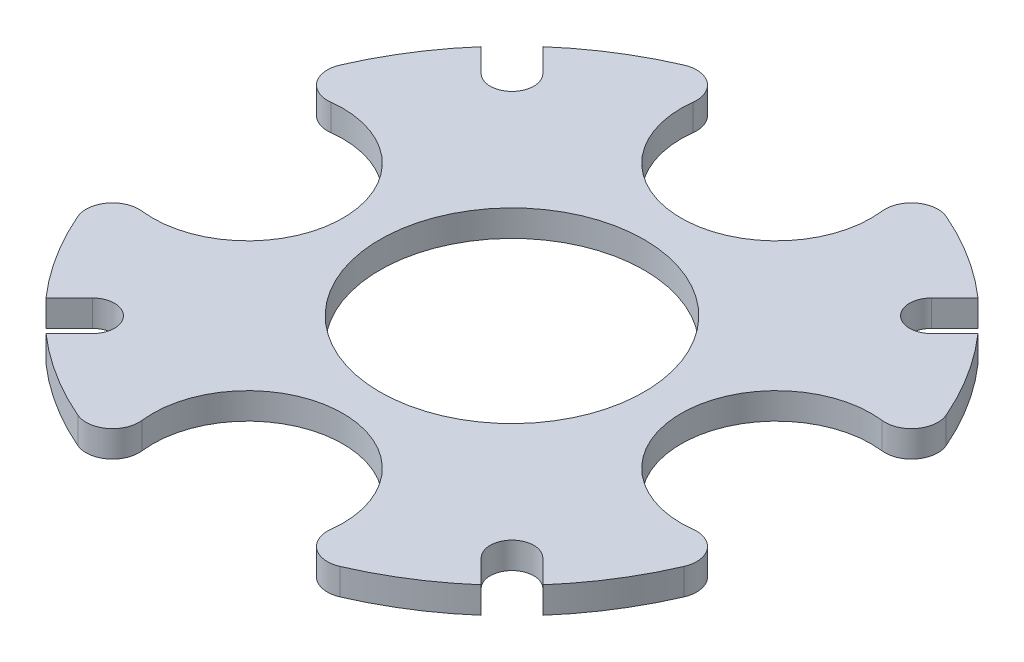
SolidWorks part; units mm, degrees
material "201 退火不锈钢 (SS)"
ref_plane "Front Plane" through (0, 0, 0) normal (0, 0, 1) x (1, 0, 0)
ref_plane "Top Plane" through (0, 0, 0) normal (0, 1, 0) x (1, 0, 0)
ref_plane "Right Plane" through (0, 0, 0) normal (1, 0, 0) x (0, 0, -1)
sketch "Sketch4" plane through (0, 0, 0) normal (0, 1, 0) x (1, 0, 0)
  line L0 (0, 0) -> (0, -19.4098) construction
  line L1 (0, 0) -> (-8.8388, -8.8388) construction
  line L2 (-7.3539, -8.5206) -> (-8.2362, -9.4029)
  line L3 (-8.5206, -7.3539) -> (-9.4029, -8.2362)
  line L10 (-7.3539, 8.5206) -> (-8.2362, 9.4029)
  line L11 (-8.5206, 7.3539) -> (-9.4029, 8.2362)
  line L12 (0, 0) -> (42.4923, 0) construction
  line L13 (8.5206, 7.3539) -> (9.4029, 8.2362)
  line L14 (7.3539, 8.5206) -> (8.2362, 9.4029)
  line L15 (7.3539, -8.5206) -> (8.2362, -9.4029)
  line L16 (8.5206, -7.3539) -> (9.4029, -8.2362)
  arc A0 (-7.3539, -8.5206) -> (-8.5206, -7.3539) centre (-7.9373, -7.9373) ccw
  arc A4 (-8.2362, -9.4029) -> (-4.9635, -11.4723) centre (0, 0) ccw
  arc A5 (-4.9635, -11.4723) -> (-3.5737, -10.434) centre (-4.5665, -10.5545) ccw
  arc A6 (3.5737, -10.434) -> (-3.5737, -10.434) centre (0, -10) ccw
  arc A7 (3.5737, -10.434) -> (4.9635, -11.4723) centre (4.5665, -10.5545) ccw
  arc A9 (4.9635, -11.4723) -> (8.2362, -9.4029) centre (0, 0) ccw
  arc A10 (11.4723, -4.9635) -> (10.434, -3.5737) centre (10.5545, -4.5665) ccw
  arc A11 (10.434, 3.5737) -> (10.434, -3.5737) centre (10, 0) ccw
  arc A15 (4.9635, 11.4723) -> (3.5737, 10.434) centre (4.5665, 10.5545) ccw
  arc A16 (-3.5737, 10.434) -> (3.5737, 10.434) centre (0, 10) ccw
  arc A17 (-3.5737, 10.434) -> (-4.9635, 11.4723) centre (-4.5665, 10.5545) ccw
  arc A19 (-4.9635, 11.4723) -> (-8.2362, 9.4029) centre (0, 0) ccw
  arc A20 (-11.4723, 4.9635) -> (-10.434, 3.5737) centre (-10.5545, 4.5665) ccw
  arc A21 (-10.434, -3.5737) -> (-10.434, 3.5737) centre (-10, 0) ccw
  arc A22 (-10.434, -3.5737) -> (-11.4723, -4.9635) centre (-10.5545, -4.5665) ccw
  arc A23 (-11.4723, -4.9635) -> (-9.4029, -8.2362) centre (0, 0) ccw
  circle A24 centre (0, 0) radius 10 construction
  arc A26 (-9.4029, -8.2362) -> (-8.2362, -9.4029) centre (0, 0) ccw construction
  circle A27 centre (0, 0) radius 5
  arc A28 (4.9635, 11.4723) -> (8.2362, 9.4029) centre (0, 0) cw
  arc A29 (10.434, 3.5737) -> (11.4723, 4.9635) centre (10.5545, 4.5665) ccw
  arc A30 (-8.5206, 7.3539) -> (-7.3539, 8.5206) centre (-7.9373, 7.9373) ccw
  arc A31 (7.3539, 8.5206) -> (8.5206, 7.3539) centre (7.9373, 7.9373) ccw
  arc A32 (8.5206, -7.3539) -> (7.3539, -8.5206) centre (7.9373, -7.9373) ccw
  arc A33 (-9.4029, 8.2362) -> (-11.4723, 4.9635) centre (0, 0) ccw
  arc A34 (9.4029, 8.2362) -> (11.4723, 4.9635) centre (0, 0) cw
  arc A35 (9.4029, -8.2362) -> (11.4723, -4.9635) centre (0, 0) ccw
  point P56 (0, 0)
  dimension "D4" = 25
  dimension "D5" = 20
  dimension "D6" = 7.2
  dimension "D7" = 2.1
  dimension "D3" = 10
  dimension "D8" = 1
  dimension "D1" = 45
  dimension "D2" = 1.65
  dimension "D9" = 4
extrude "Boss-Extrude1" add sketch "Sketch4" along normal blind 1
